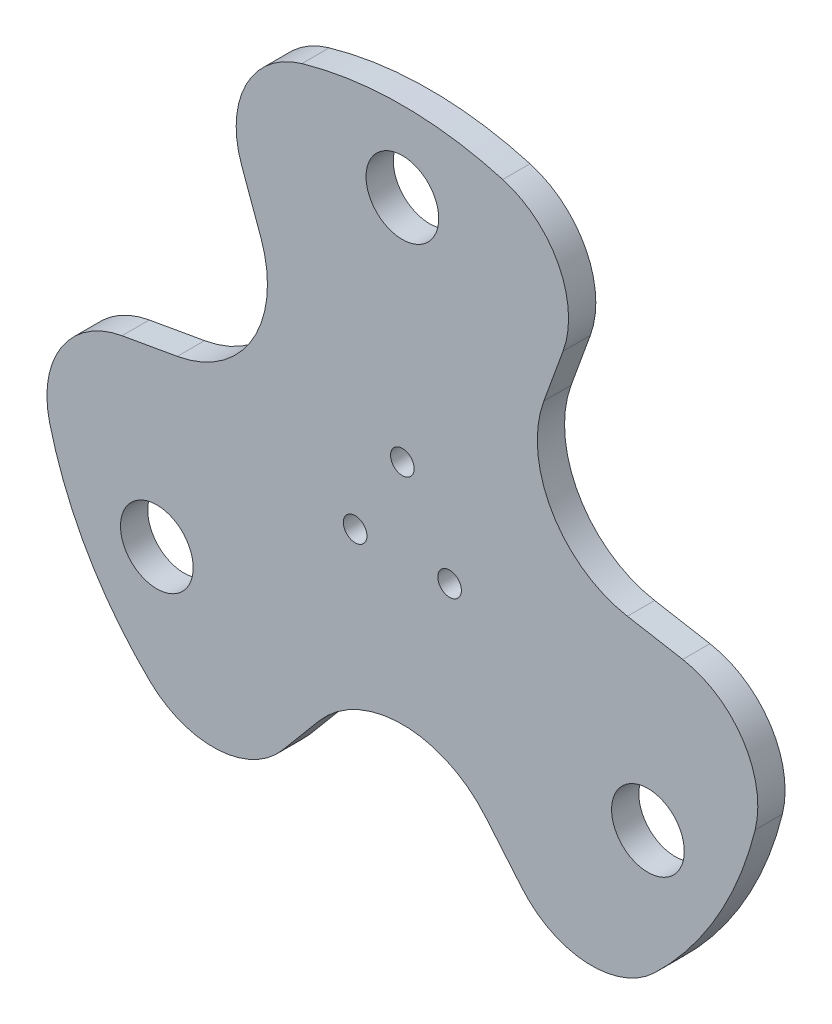
from build123d import *

# Parameters (mm, degrees)
SKETCH1_R           = 200
SKETCH1_R_2         = 20
BOSS_EXTRUDE1_DEPTH = 15
CUT_EXTRUDE1_DEPTH  = 30
FILLET1_R           = 50
SKETCH3_R           = 6.5
CUT_EXTRUDE2_DEPTH  = 50


with BuildPart() as part:
    # Sketch1 → Boss-Extrude1 (new body)
    with BuildSketch(Plane.XY):
        Circle(SKETCH1_R)
        with Locations((0, 156)):
            Circle(SKETCH1_R_2, mode=Mode.SUBTRACT)
        with Locations((135.09996299, -78)):
            Circle(SKETCH1_R_2, mode=Mode.SUBTRACT)
        with Locations((-135.09996299, -78)):
            Circle(SKETCH1_R_2, mode=Mode.SUBTRACT)
    extrude(amount=BOSS_EXTRUDE1_DEPTH)

    # Sketch2 → Cut-Extrude1 (cut)
    with BuildSketch(Plane.XY.offset(15)):
        with BuildLine():
            Line((-45.962666587, -116.432743419), (-177.651298468, -273.373143566))
            Line((-177.651298468, -273.373143566), (100.686015144, -181.64949066))
            Line((100.686015144, -181.64949066), (45.962666587, -116.432743419))
            ThreePointArc((45.962666587, -116.432743419), (0, -95), (-45.962666587, -116.432743419))
        make_face()
        with BuildLine():
            Line((-77.852380339, 98.0212086), (-147.922437807, 290.537109271))
            Line((-147.922437807, 290.537109271), (-207.656081069, 3.62809841))
            Line((-207.656081069, 3.62809841), (-123.815046927, 18.411534819))
            ThreePointArc((-123.815046927, 18.411534819), (-82.27241336, 47.5), (-77.852380339, 98.0212086))
        make_face()
        with BuildLine():
            Line((123.815046927, 18.411534819), (325.573736275, -17.163965705))
            Line((325.573736275, -17.163965705), (106.970065924, 178.021392251))
            Line((106.970065924, 178.021392251), (77.852380339, 98.0212086))
            ThreePointArc((77.852380339, 98.0212086), (82.27241336, 47.5), (123.815046927, 18.411534819))
        make_face()
    extrude(amount=-CUT_EXTRUDE1_DEPTH, mode=Mode.SUBTRACT)

    # Fillet1
    fillet1_edges = [part.edges().sort_by_distance(p)[0] for p in [
        (199.937763867, 4.989045978, 7.5),
        (104.289522491, 170.656659696, 7.5),
        (-104.289522491, 170.656659696, 7.5),
        (-199.937763867, 4.989045978, 7.5),
        (-95.648241376, -175.645705674, 7.5),
        (95.648241376, -175.645705674, 7.5),
    ]]
    fillet(fillet1_edges, radius=FILLET1_R)

    # Sketch3 → Cut-Extrude2 (cut)
    with BuildSketch(Plane.XY.offset(15)):
        with Locations((0, 30)):
            Circle(SKETCH3_R)
        with Locations((25.980762114, -15)):
            Circle(SKETCH3_R)
        with Locations((-25.980762114, -15)):
            Circle(SKETCH3_R)
    extrude(amount=-CUT_EXTRUDE2_DEPTH, mode=Mode.SUBTRACT)


solid = part.part
